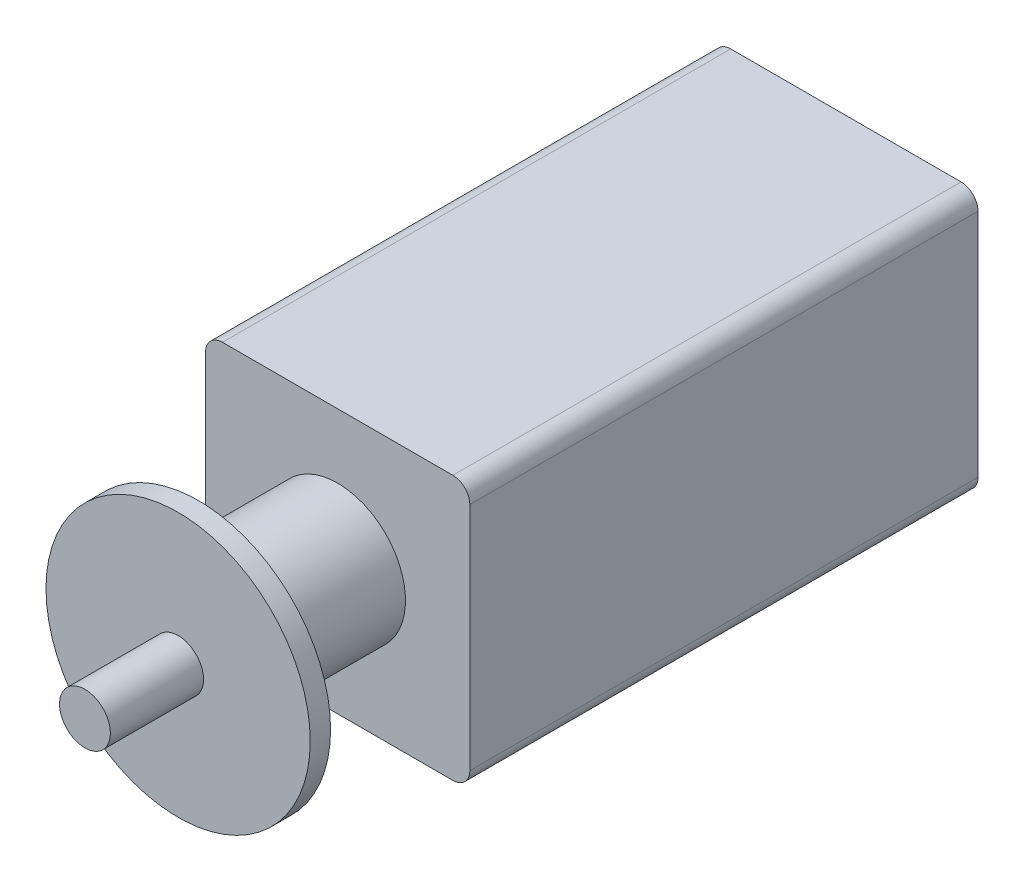
SolidWorks part; units mm, degrees
ref_plane "Front Plane" through (0, 0, 0) normal (0, 0, 1) x (1, 0, 0)
ref_plane "Top Plane" through (0, 0, 0) normal (0, 1, 0) x (1, 0, 0)
ref_plane "Right Plane" through (0, 0, 0) normal (1, 0, 0) x (0, 0, -1)
sketch "Sketch1" plane through (0, 0, 0) normal (0, 0, 1) x (1, 0, 0)
  line L1 (0, 0) -> (156, 0)
  line L2 (0, 0) -> (0, 156)
  line L3 (0, 156) -> (156, 156)
  line L4 (156, 0) -> (156, 156)
  dimension "D1" = 156
  dimension "D2" = 156
extrude "Boss-Extrude1" add sketch "Sketch1" along normal blind 300
sketch "Sketch2" plane through (0, 0, 300) normal (0, 0, 1) x (1, 0, 0)
  circle A0 centre (78, 78) radius 40
  dimension "D1" = 80
extrude "Boss-Extrude2" add sketch "Sketch2" along normal blind 88
sketch "Sketch3" plane through (0, 0, 388) normal (0, 0, 1) x (1, 0, 0)
  circle A0 centre (83.7881, 78) radius 78
  dimension "D1" = 156
extrude "Boss-Extrude3" add sketch "Sketch3" along normal blind 12
fillet "Fillet1" radius 10 4 edges at (156, 0, 150) (0, 0, 150) (156, 156, 150) (0, 156, 150)
sketch "Sketch4" plane through (0, 0, 400) normal (0, 0, 1) x (1, 0, 0)
  circle A0 centre (83.7881, 78) radius 15
  dimension "D1" = 30
extrude "Boss-Extrude4" add sketch "Sketch4" along normal blind 55
